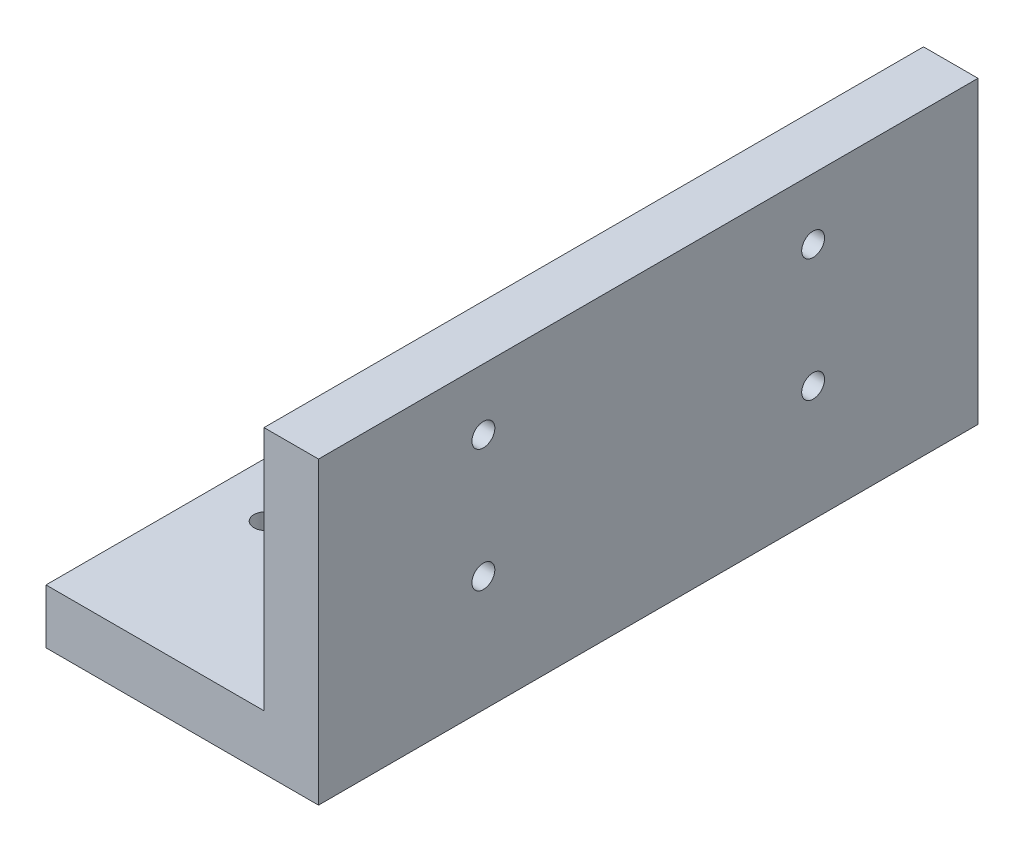
SolidWorks part; units mm, degrees
ref_plane "前视基准面" through (0, 0, 0) normal (0, 0, 1) x (1, 0, 0)
ref_plane "上视基准面" through (0, 0, 0) normal (0, 1, 0) x (1, 0, 0)
ref_plane "右视基准面" through (0, 0, 0) normal (1, 0, 0) x (0, 0, -1)
sketch "草图1" plane through (0, 0, 0) normal (0, 0, 1) x (1, 0, 0)
  line L0 (0, 24.5105) -> (10, 24.5105)
  line L1 (10, 24.5105) -> (10, -30.4895)
  line L2 (10, -30.4895) -> (-40, -30.4895)
  line L3 (-40, -30.4895) -> (-40, -20.4895)
  line L4 (-40, -20.4895) -> (0, -20.4895)
  line L5 (0, -20.4895) -> (0, 24.5105)
  dimension "D1" = 10
  dimension "D2" = 40
  dimension "D3" = 45
  dimension "D4" = 10
extrude "凸台-拉伸1" add sketch "草图1" along normal blind 121
extrude "切除-拉伸2" cut sketch "草图3" against normal up to surface (25 mm away)
sketch "草图3" plane through (-858.744, -20.4895, -869.1439) normal (0, 1, 0) x (-1, 0, 0)
  line L1 (-838.744, 990.1439) -> (-858.744, 990.1439) construction
  line L3 (-848.744, 990.1439) -> (-848.744, 869.1439) construction
  line L5 (-838.744, 990.1439) -> (-818.744, 990.1439) construction
  line L6 (-828.744, 990.1439) -> (-828.744, 869.1439) construction
  line L7 (-818.744, 929.6439) -> (-818.744, 869.1439) construction
  line L9 (-818.744, 899.3939) -> (-858.744, 899.3939) construction
  line L11 (-818.744, 990.1439) -> (-818.744, 929.6439) construction
  line L12 (-818.744, 959.8939) -> (-858.744, 959.8939) construction
  circle A0 centre (-848.744, 959.8939) radius 2.1
  circle A1 centre (-828.744, 959.8939) radius 2.1
  circle A2 centre (-828.744, 899.3939) radius 2.1
  circle A3 centre (-848.744, 899.3939) radius 2.1
sketch "草图4" plane through (0, -20.4895, 0) normal (0, 1, 0) x (1, 0, 0)
  circle A0 centre (-30, -30.25) radius 2.1
  circle A1 centre (-10, -30.25) radius 2.1
  circle A2 centre (-30, -90.75) radius 2.1
  circle A3 centre (-10, -90.75) radius 2.1
sketch "草图5" plane through (0, 0, 0) normal (-1, 0, 0) x (0, 0, 1)
  circle A0 centre (30.25, 13.2605) radius 2.1
  circle A1 centre (30.25, -9.2395) radius 2.1
  circle A2 centre (90.75, 13.2605) radius 2.1
  circle A3 centre (90.75, -9.2395) radius 2.1
extrude "切除-拉伸3" cut sketch "草图5" against normal up to surface (10 mm away) up to face at (10, -2.9895, 60.5)
